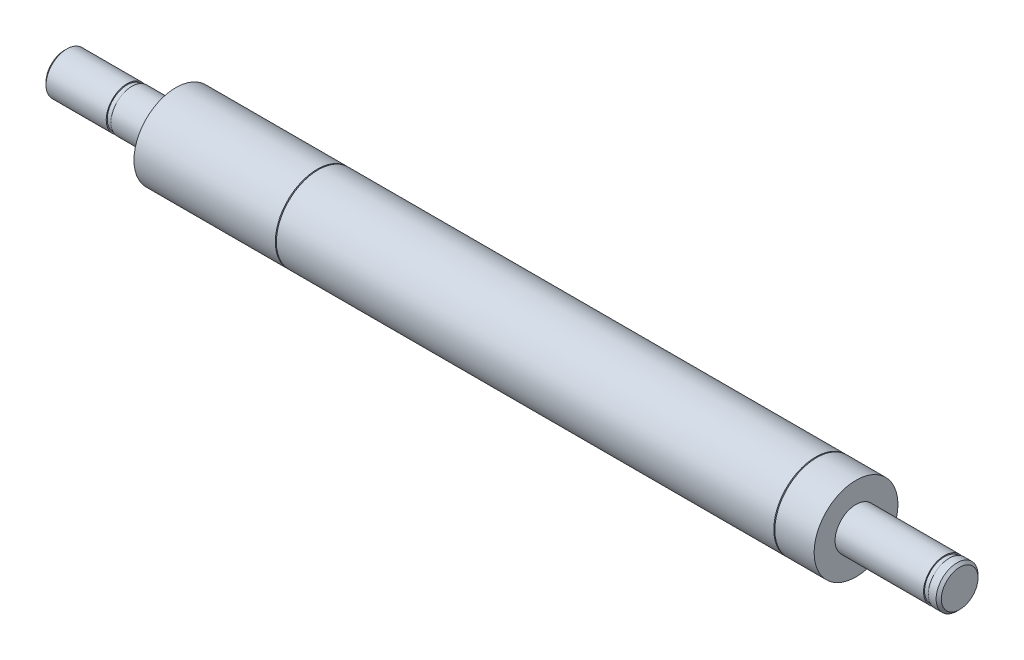
SolidWorks part; units mm, degrees
ref_plane "Front" through (0, 0, 0) normal (0, 0, 1) x (1, 0, 0)
ref_plane "Top" through (0, 0, 0) normal (0, 1, 0) x (1, 0, 0)
ref_plane "Right" through (0, 0, 0) normal (1, 0, 0) x (0, 0, -1)
sketch "Sketch1" plane through (0, 0, 0) normal (0, 1, 0) x (1, 0, 0)
  line L0 (-12.2567, 0) -> (181.8764, 0) construction
  line L1 (0, 0) -> (0, -4)
  line L2 (0, -4) -> (21.3, -4)
  line L5 (21.3, -4) -> (21.3, -8)
  line L6 (21.3, -8) -> (151.2, -8)
  line L7 (151.2, -8) -> (151.2, -4)
  line L8 (151.2, -4) -> (171, -4)
  line L9 (171, -4) -> (171, 0)
  line L10 (171, 0) -> (0, 0)
  dimension "D1" = 19.8
  dimension "D2" = 129.9
  dimension "D3" = 8
  dimension "D4" = 21.3
  dimension "D7" = 16
  dimension "D8" = 8
revolve "Revolve1" add sketch "Sketch1" angle 360 mid plane about L0
sketch "Sketch2" plane through (0, 0, 0) normal (0, 1, 0) x (1, 0, 0)
  line L0 (-6.3552, 0) -> (198.6277, 0) construction
  line L1 (21.3, -8) -> (151.2, -8) construction
  line L2 (48.3, -8) -> (48.5, -8)
  line L3 (48.3, -8) -> (48.3, -6.4)
  line L4 (48.3, -6.4) -> (48.5, -6.4)
  line L5 (48.5, -8) -> (48.5, -6.4)
  line L6 (21.3, -8) -> (151.2, -8) construction
  line L7 (143.5, -8) -> (143.7, -8)
  line L8 (143.5, -8) -> (143.5, -6.4)
  line L9 (143.5, -6.4) -> (143.7, -6.4)
  line L10 (143.7, -8) -> (143.7, -6.4)
  line L11 (151.2, -4) -> (171, -4) construction
  line L12 (168.1, -4) -> (169, -4)
  line L13 (168.1, -4) -> (168.1, -3.8)
  line L14 (168.1, -3.8) -> (169, -3.8)
  line L15 (169, -4) -> (169, -3.8)
  line L16 (0, -4) -> (21.3, -4) construction
  line L17 (12, -4) -> (12.9, -4)
  line L18 (12, -4) -> (12, -3.8)
  line L19 (12, -3.8) -> (12.9, -3.8)
  line L20 (12.9, -4) -> (12.9, -3.8)
  dimension "D1" = 12
  dimension "D2" = 0.2
  dimension "D3" = 95
  dimension "D4" = 12.8
  dimension "D5" = 24.6
  dimension "D6" = 0.9
  dimension "D7" = 7.6
  dimension "D8" = 36.5
revolve "Cut-Revolve1" cut sketch "Sketch2" angle 360 mid plane about L0
chamfer "Chamfer1" distance 0.5 angle 45 2 edges at (0, 0, 4) (171, 0, 4)
